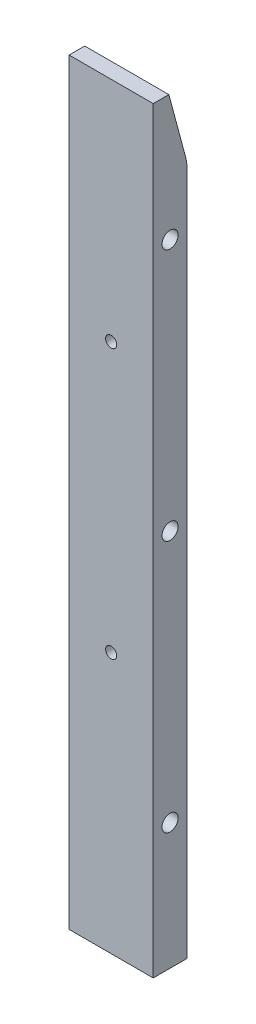
SolidWorks part; units mm, degrees
material "电木（PF）"
ref_plane "前视基准面" through (0, 0, 0) normal (0, 0, 1) x (1, 0, 0)
ref_plane "上视基准面" through (0, 0, 0) normal (0, 1, 0) x (1, 0, 0)
ref_plane "右视基准面" through (0, 0, 0) normal (1, 0, 0) x (0, 0, -1)
sketch "草图1" plane through (0, 0, 0) normal (1, 0, 0) x (0, 0, -1)
  line L1 (-5, 112.5) -> (5, 112.5)
  line L2 (-5, 112.5) -> (-5, -112.5)
  line L3 (-5, -112.5) -> (5, -112.5)
  line L4 (5, 112.5) -> (5, -112.5)
  line L5 (-5, 112.5) -> (5, -112.5) construction
  line L6 (-5, -112.5) -> (5, 112.5) construction
  point P0 (0, 0)
  dimension "D1" = 10
  dimension "D2" = 225
extrude "凸台-拉伸1" add sketch "草图1" along normal mid plane 25
chamfer "倒角1" distance 20 angle 15 1 edges at (0, 112.5, -5)
hole_wizard "打孔尺寸(%根据)开槽圆柱头螺钉的类型1" positions "草图2" profile "草图4" counterbore size "M4" standard "GB" end condition through all
sketch "草图2" plane through (-12.5, 0, 0) normal (-1, 0, 0) x (0, 0, 1)
  line L0 (0, 0) -> (68.9377, 0) construction
  point P0 (0, 75)
  point P2 (0, 0)
  point P5 (0, -75)
  dimension "D1" = 150
sketch "草图4" plane through (-12.5, 75, 0) normal (0, 1, 0) x (0, 0, 1)
  line L0 (0, 0) -> (0, 25)
  line L1 (0, 25) -> (2.4, 25)
  line L3 (2.4, 25) -> (2.4, 5)
  line L4 (2.4, 5) -> (4, 5)
  line L5 (4, 5) -> (4, 0)
  line L7 (4, 0) -> (0, 0)
  line L11 (0, -6.35) -> (0, 107.95) construction
  dimension "通孔孔直径" = 4.8
  dimension "通孔孔深度" = 25
  dimension "柱形沉头孔直径" = 8
  dimension "柱形沉头孔深度" = 5
chamfer "倒角2" [suppressed] distance 20 angle 15
hole_wizard "M4 螺纹孔1" positions "草图5" profile "草图6" tap size "M4" standard "GB" end condition through all
sketch "草图5" plane through (0, 0, 5) normal (0, 0, 1) x (1, 0, 0)
  point P0 (0, 45)
  point P3 (0, -35)
sketch "草图6" plane through (0, 45, 5) normal (1, 0, 0) x (0, -1, 0)
  line L0 (0, 0) -> (0, 10)
  line L1 (0, 10) -> (1.65, 10)
  line L2 (1.65, 10) -> (1.65, 0)
  line L5 (1.65, 0) -> (0, 0)
  line L11 (0, -6.35) -> (0, 107.95) construction
  dimension "通孔螺纹孔钻头直径" = 3.3
  dimension "通孔螺纹孔钻头深度" = 10
cosmetic thread "孔螺蚊线1" parameters "D2"=4
cosmetic thread "孔螺蚊线2" parameters "D2"=4
fillet "圆角1" radius 10 1 edges at (0, 92.5, -5)
